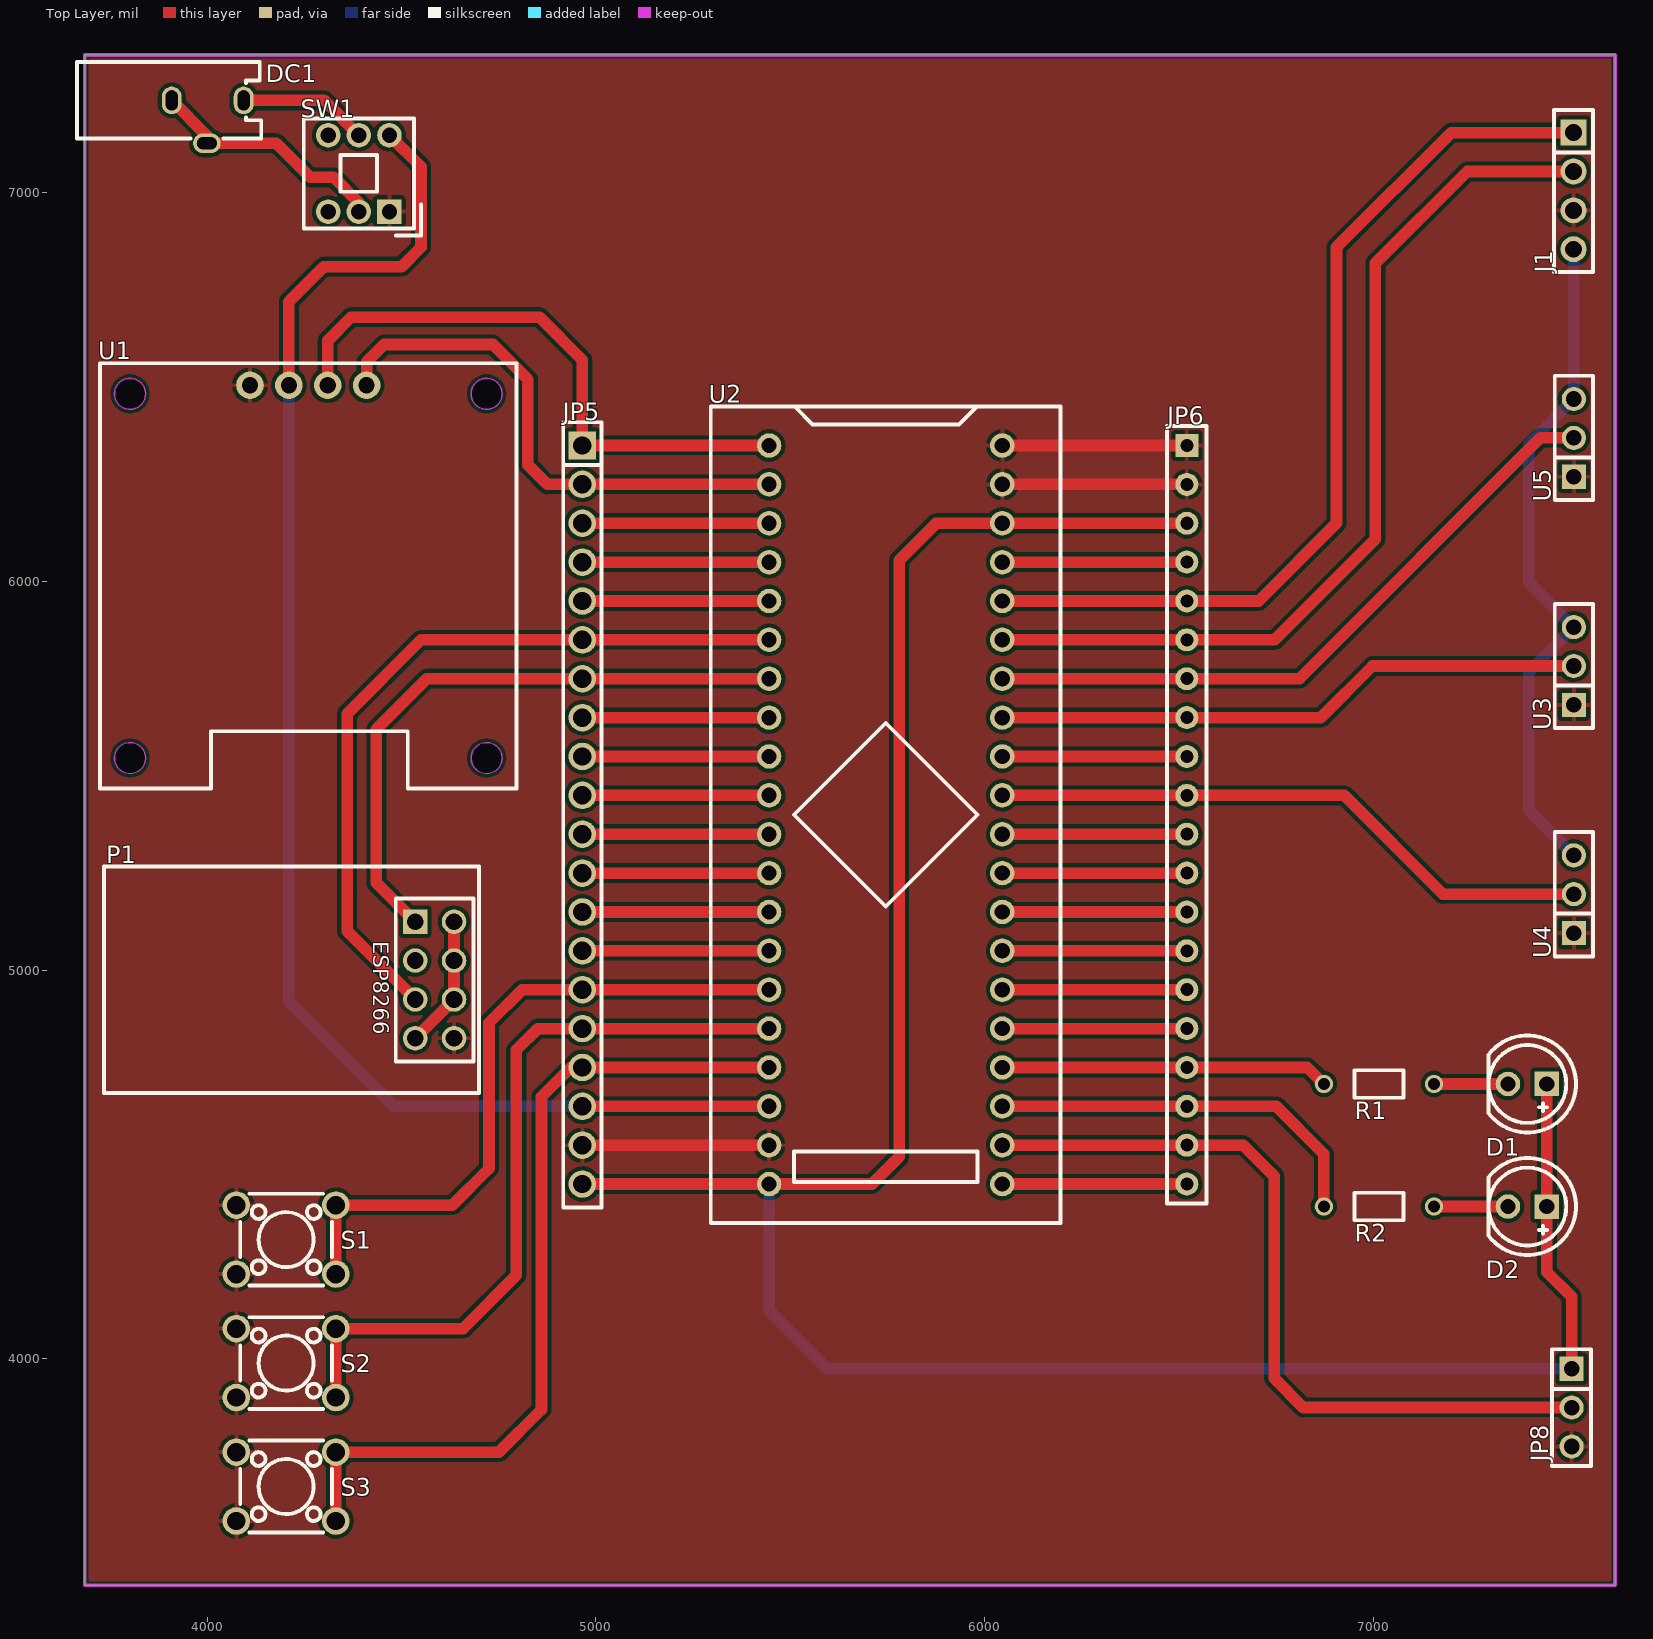
[diagram p0: Top Layer view]
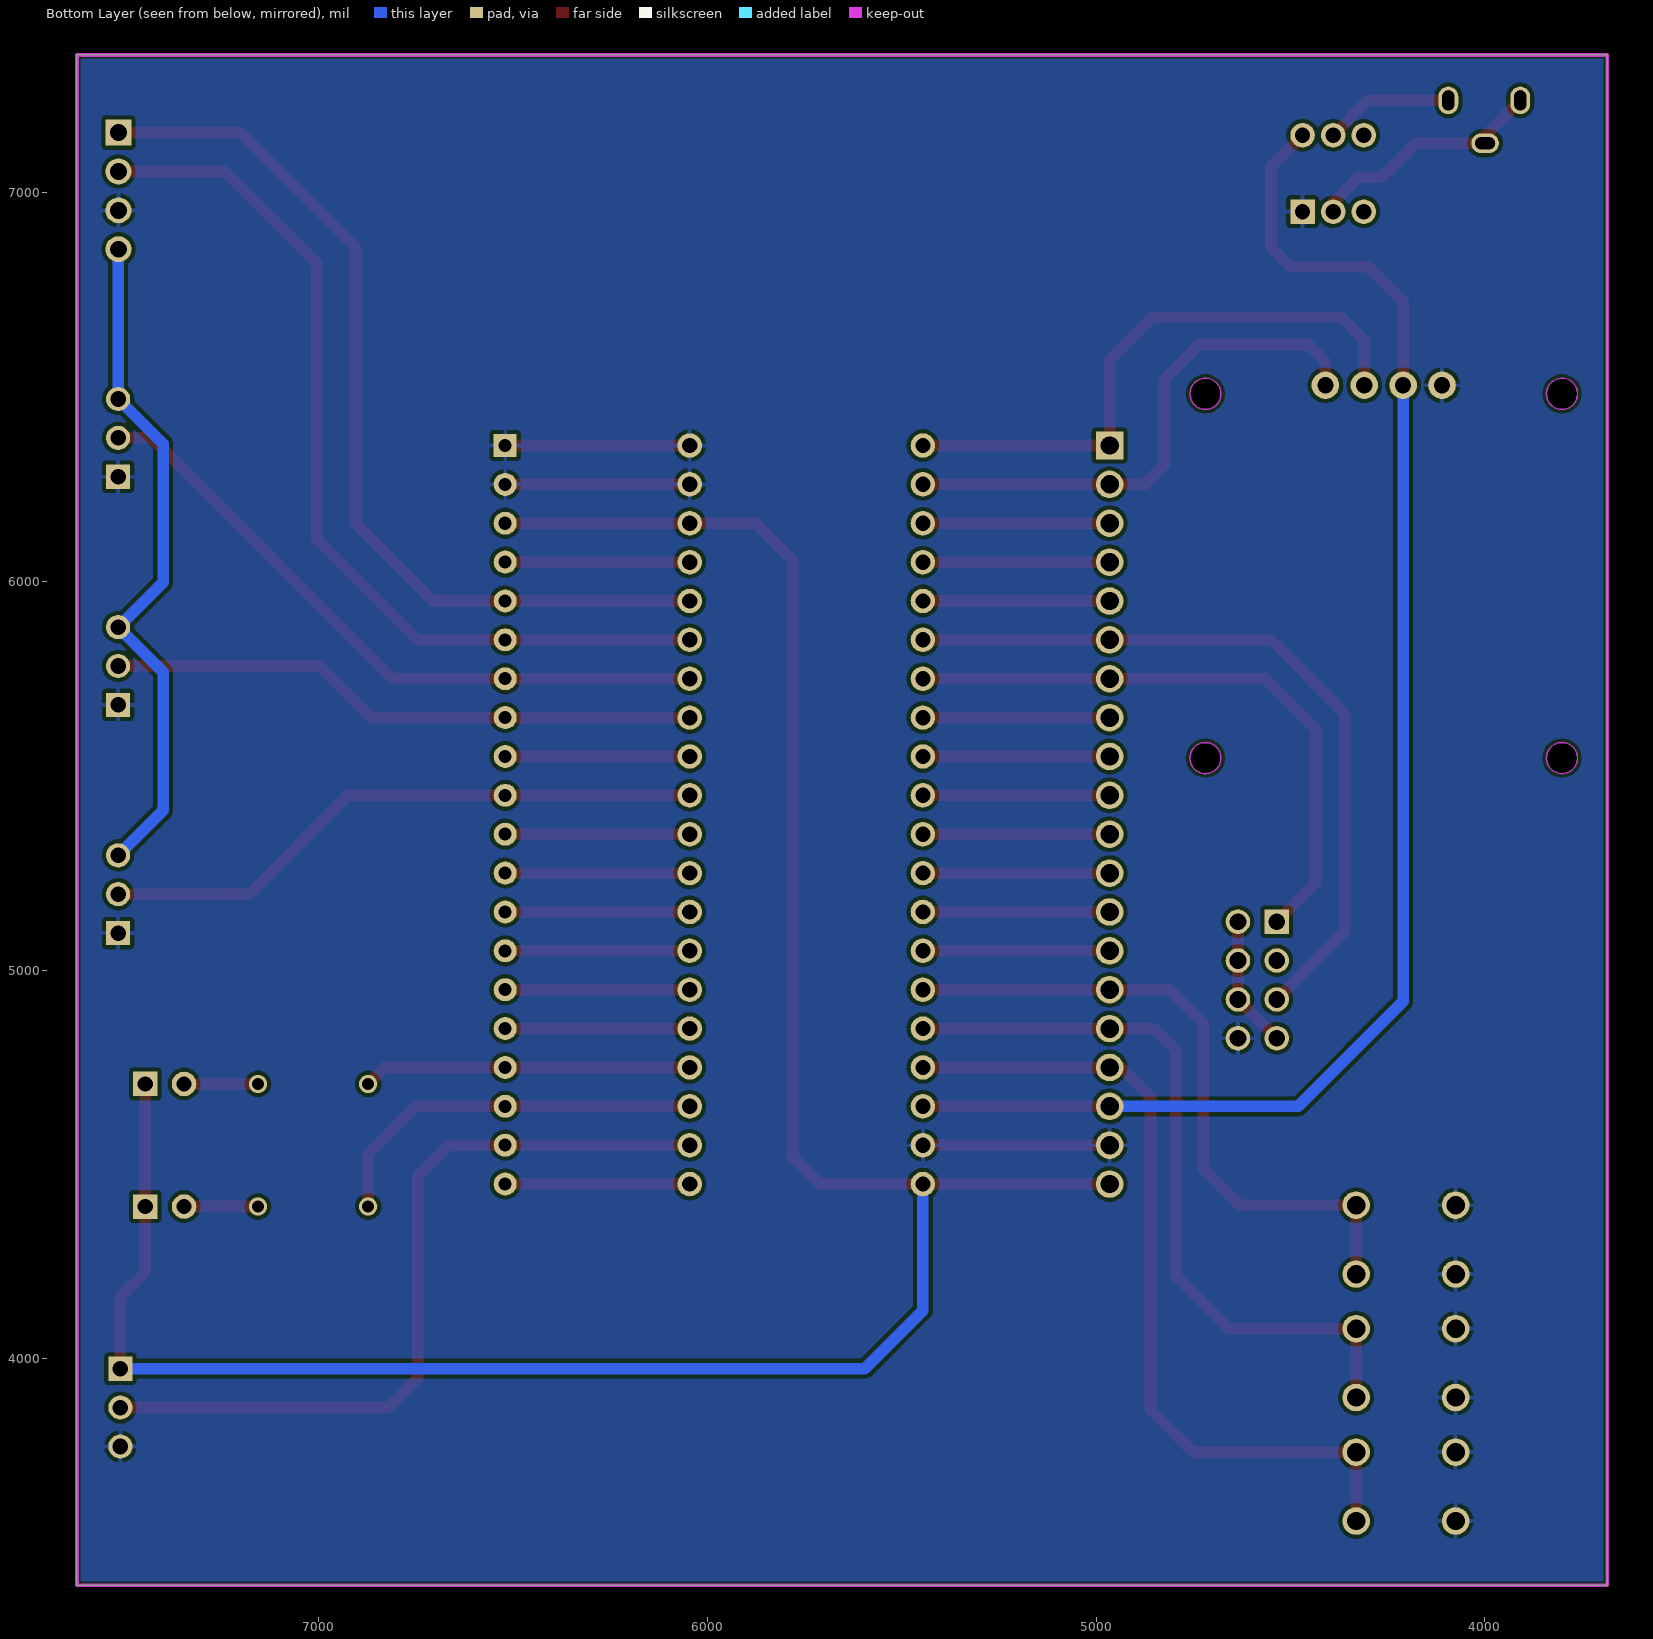
[diagram p1: Bottom Layer view, seen from below]
# Altium PCB MISC61251.pcbdoc
Units mil, origin at the board's own origin, x right, y up, seen from the top; angles counter-clockwise.
Board outline 3937.01 x 3937.01 mil, 2 copper layers (Top Layer, Bottom Layer), stack 62.206 mil thick; 19 components, 43 nets, 137 pads, 0 vias.

## Layer stack, top to bottom
Top Solder Mask Layer: solder mask 0.394, Dk 3.3
Top Layer: signal copper 1.379
Dielectric1: surface 59.449, FR4, Dk 4.5
Bottom Layer: signal copper 1.378
Bottom Solder Mask Layer: solder mask 0.394, Dk 3.3

## Board outline
3685,7355 3685,3417.99 7622.01,3417.99 7622.01,7355

## Design rules (kind name [scope] priority, off if disabled: settings)
BoardOutlineClearance copperThickness2oz_1 [All] p2 off: genericclearance=7.99 ignorepadtopadclearanceinfootprint=FALSE except(0: Arc-SplitContinuation Track-SplitContinuation SMDPad-SplitContinuation THPad-SplitContinuation Via-SplitContinuation Fill-SplitContinuation Region-SplitContinuation Poly-SplitContinuation Text-SplitContinuation Hole-SplitContinuation; 5.98: Arc-CutoutEdge SMDPad-CutoutEdge THPad-CutoutEdge Via-CutoutEdge Fill-CutoutEdge Region-CutoutEdge Text-CutoutEdge; 6.93: Hole-OutlineEdge Hole-CutoutEdge; 10: Poly-OutlineEdge Poly-CutoutEdge; 11.81: Arc-OutlineEdge Track-OutlineEdge SMDPad-OutlineEdge THPad-OutlineEdge Via-OutlineEdge Fill-OutlineEdge Region-OutlineEdge Text-OutlineEdge Track-CutoutEdge)
BoardOutlineClearance copperThickness1oz_1 [All] p4: genericclearance=4.02 ignorepadtopadclearanceinfootprint=FALSE except(0: Arc-SplitContinuation Track-SplitContinuation SMDPad-SplitContinuation THPad-SplitContinuation Via-SplitContinuation Fill-SplitContinuation Region-SplitContinuation Poly-SplitContinuation Text-SplitContinuation Hole-SplitContinuation; 6: SMDPad-CutoutEdge THPad-CutoutEdge Via-CutoutEdge Fill-CutoutEdge Region-CutoutEdge Text-CutoutEdge; 6.93: Hole-OutlineEdge Hole-CutoutEdge; 10: Poly-OutlineEdge Poly-CutoutEdge; 11.8: Arc-OutlineEdge Track-OutlineEdge SMDPad-OutlineEdge THPad-OutlineEdge Via-OutlineEdge Fill-OutlineEdge Region-OutlineEdge Text-OutlineEdge; 11.81: Arc-CutoutEdge Track-CutoutEdge)
Clearance copperThickness2oz [All] p1 off: gap=7.99 ignorepadtopadclearanceinfootprint=FALSE except(5.98: SMDPad-Track SMDPad-SMDPad THPad-Track SMDPad-THPad THPad-THPad Track-Via SMDPad-Via THPad-Via Via-Via Fill-Track Region-Track Fill-SMDPad Region-SMDPad Fill-THPad Region-THPad Fill-Via Region-Via Fill-Fill Fill-Region Region-Region Arc-Track Arc-SMDPad Arc-THPad Arc-Via Fill-Arc Region-Arc Arc-Arc Text-Track SMDPad-Text Text-THPad Text-Via Fill-Text Region-Text Arc-Text Text-Text; 6.93: Hole-Track Hole-SMDPad Hole-THPad Hole-Via Fill-Hole Region-Hole Hole-Arc Hole-Text; 10: Poly-Track Poly-SMDPad Poly-THPad Poly-Via Poly-Fill Poly-Region Poly-Poly Poly-Arc Poly-Text Poly-Hole)
Clearance copperThickness1oz [All] p3: gap=4.02 ignorepadtopadclearanceinfootprint=FALSE except(5.98: SMDPad-Track SMDPad-SMDPad THPad-Track SMDPad-THPad THPad-THPad Track-Via SMDPad-Via THPad-Via Via-Via Fill-Track Region-Track Fill-SMDPad Region-SMDPad Fill-THPad Region-THPad Fill-Via Region-Via Fill-Fill Fill-Region Region-Region; 6: Arc-Track Arc-SMDPad Arc-THPad Arc-Via Fill-Arc Region-Arc Arc-Arc Text-Track SMDPad-Text Text-THPad Text-Via Fill-Text Region-Text Arc-Text Text-Text; 6.93: Hole-Track Hole-SMDPad Hole-THPad Hole-Via Fill-Hole Region-Hole Hole-Arc Hole-Text; 10: Poly-Track Poly-SMDPad Poly-THPad Poly-Via Poly-Fill Poly-Region Poly-Poly Poly-Arc Poly-Text Poly-Hole)
DiffPairsRouting differentialPair [All] p1: maxlimit=6 minlimit=6 mostfreqgap=6 toplayer_minwidth=5 toplayer_prefwidth=10 toplayer_maxwidth=100 toplayer_mingap=6 toplayer_prefgap=6 toplayer_maxgap=6 bottomlayer_minwidth=5 bottomlayer_prefwidth=10 bottomlayer_maxwidth=100 bottomlayer_mingap=6 bottomlayer_prefgap=6 bottomlayer_maxgap=6 maxuncoupledlength=10
HoleToHoleClearance otherClearance [All] p1: gap=11.81 allowstackedmicrovias=TRUE
Length netLength [All] p1: minlimit=0 maxlimit=0
MatchedLengths netLengthTolerance [All] p1: tolerance=1000
PasteMaskExpansion pasteMaskExpansion [All] p1: expansion=0
PlaneConnect innerPlane [All] p1: planeconnectstyle=Relief reliefexpansion=20 reliefentries=4 reliefconductorwidth=10 reliefairgap=10
PolygonConnect copperRegion [(InNet('GND'))] p1: connectstyle=Relief reliefconductorwidth=10 reliefentries=4 polygonreliefangle="90 Angle" airgapwidth=10 via.connectstyle=Relief via.reliefconductorwidth=10 via.reliefentries=4 via.polygonreliefangle="90 Angle" via.airgapwidth=10
RoutingVias viaSize [All] p1: holewidth=12.01 width=24.02 viastyle="Through Hole" minholewidth=11.81 minwidth=19.68 maxholewidth=248.03 maxwidth=393.7
SolderMaskExpansion solderMaskExpansion [IsVia] p1: expansion=-1000 istentingtop=TRUE
SolderMaskExpansion solderMaskExpansion [All] p2: expansion=2 istentingtop=FALSE
Width copperThickness2oz_2 [All] p1 off: maxlimit=100 minlimit=8 preferedwidth=10
Width copperThickness1oz_2 [All] p2: maxlimit=100 minlimit=5 preferedwidth=10

## Components (designator, comment, footprint, x,y, rotation, side; value= is the part's Value field where it differs from the comment)
D1 "led" LED-TH_5mm 7396.22,4707.52 r180 top
D2 "led" LED-TH_5mm 7396.22,4392.2 r180 top
DC1 "DC002-1.3" DC-IN-TH_DC002-1.3 4001.22,7182.72 r270 top
J1 "" HDR-TH_4P-P2.54-V-F 7515,7005 r270 top
JP5 "HDR-1X20" HDR-TH_20P-P2.54-V-F 4965,5400 r270 top
JP6 "HDR-1X20" HDR-TH_20P-P2.54-V-F-6 6520,5400 r270 top
JP8 "HDR-1X3" HDR-TH_3P-P2.54-V-F-4 7510,3875 r270 top
P1 "" ESP8266-1 4585,4975 r270 top
R1 "Res2" Res_1/8W 7014.4,4709.99 r180 top
R2 "Res2" Res_1/8W 7014.4,4394.68 r180 top
S1 "key_4" SW-TH_4P-L6.0-W6.0-P4.50-LS6.5 4203.02,4307.03 r180 top
S2 "key_4" SW-TH_4P-L6.0-W6.0-P4.50-LS6.5 4203.02,3989.4 r180 top
S3 "key_4" SW-TH_4P-L6.0-W6.0-P4.50-LS6.5 4203.02,3671.76 r180 top
SW1 "Self-lock button" SW-TH_6P-L7.0-W7.0-P2.00 4390,7050 r270 top
U1 "OLED" OLED-TH_L27.8-W27.2-P2.54_C9900033791 4260,6505 r0 top
U2 "ST32F103C8T6" CONN-TH_L53.3-W22.9_STM32F103C8T6-CARD 5745.45,5400 r270 top
U3 "" HDR-TH_3P-P2.54-V-F 7515.79,5782.68 r90 top
U4 "" HDR-TH_3P-P2.54-V-F 7515.79,5195.73 r90 top
U5 "DHT11" HDR-TH_3P-P2.54-V-F 7515.79,6369.63 r90 top

## Footprints (in the part's own frame and the unit in brackets; to place one, negate y for a bottom-side part, rotate by r counter-clockwise, add the part's x,y. Pads: shape width x height; smd on the part's side, far side on the other; paste and mask are expansions set on the pad)
CONN-TH_L53.3-W22.9_STM32F103C8T6-CARD [mm]
  round 1.6 hole 1: 1(-24.13,-7.62) 2(-21.59,-7.62) 3(-19.05,-7.62) 4(-16.51,-7.62) 5(-13.97,-7.62) 6(-11.43,-7.62) 7(-8.89,-7.62) 8(-6.35,-7.62) 9(-3.81,-7.62) 10(-1.27,-7.62) 11(1.27,-7.62) 12(3.81,-7.62) 13(6.35,-7.62) 14(8.89,-7.62) 15(11.43,-7.62) 16(13.97,-7.62) 17(16.51,-7.62) 18(19.05,-7.62) 19(21.59,-7.62) 20(24.13,-7.62) 21(24.13,7.62) 22(21.59,7.62) 23(19.05,7.62) 24(16.51,7.62) 25(13.97,7.62) 26(11.43,7.62) 27(8.89,7.62) 28(6.35,7.62) 29(3.81,7.62) 30(1.27,7.62) 31(-1.27,7.62) 32(-3.81,7.62) 33(-6.35,7.62) 34(-8.89,7.62) 35(-11.43,7.62) 36(-13.97,7.62) 37(-16.51,7.62) 38(-19.05,7.62) 39(-21.59,7.62) 40(-24.13,7.62)
  silkscreen extent -26.67,-11.43 26.67,11.43
DC-IN-TH_DC002-1.3 [mm]
  oval 1.8x1.3 hole 0.8 slot 1.3 at 0 deg paste+0 mask+0.05: 1(-1.4,2.35) 3(-1.4,-2.35)
  oval 1.3x1.8 hole 0.8 slot 1.3 at 90 deg paste+0 mask+0.05: 2(1.4,-0.05)
  silkscreen extent -3.9,-8.55 1.1,3.5
ESP8266-1 [mm]
  rect 1.6x1.6 hole 1.1: 1(-3.81,-1.27)
  round 1.6 hole 1.1: 2(-3.81,1.27) 3(-1.27,-1.27) 4(-1.27,1.27) 5(1.27,-1.27) 6(1.27,1.27) 7(3.81,-1.27) 8(3.81,1.27)
  silkscreen extent -7.42,-21.6 7.38,2.9
HDR-TH_3P-P2.54-V-F [mil]
  rect 62x62 hole 40.16: 1(-100,0)
  round 62 hole 40.16: 2(0,0) 3(100,0)
  silkscreen extent -160,-49 160,49
HDR-TH_3P-P2.54-V-F-4 [mil]
  rect 62x62 hole 40.16: 1(-100,0)
  round 62 hole 40.16: 2(0,0) 3(100,0)
  silkscreen extent -150,-50 150,50
HDR-TH_4P-P2.54-V-F [mm]
  rect 1.7x1.7 hole 1.1: 1(-3.81,0)
  round 1.7 hole 1.1: 2(-1.27,0) 3(1.27,0) 4(3.81,0)
  silkscreen extent -5.29,-1.27 5.29,1.27
HDR-TH_20P-P2.54-V-F [mm]
  rect 1.8x1.8 hole 1.2: 1(-24.13,0)
  round 1.8 hole 1.2: 2(-21.59,0) 3(-19.05,0) 4(-16.51,0) 5(-13.97,0) 6(-11.43,0) 7(-8.89,0) 8(-6.35,0) 9(-3.81,0) 10(-1.27,0) 11(1.27,0) 12(3.81,0) 13(6.35,0) 14(8.89,0) 15(11.43,0) 16(13.97,0) 17(16.51,0) 18(19.05,0) 19(21.59,0) 20(24.13,0)
  silkscreen extent -25.65,-1.25 25.65,1.25
HDR-TH_20P-P2.54-V-F-6 [mm]
  rect 1.5x1.5 hole 0.85 paste+0 mask+0.05: 1(-24.13,0)
  round 1.5 hole 0.85 paste+0 mask+0.05: 2(-21.59,0) 3(-19.05,0) 4(-16.51,0) 5(-13.97,0) 6(-11.43,0) 7(-8.89,0) 8(-6.35,0) 9(-3.81,0) 10(-1.27,0) 11(1.27,0) 12(3.81,0) 13(6.35,0) 14(8.89,0) 15(11.43,0) 16(13.97,0) 17(16.51,0) 18(19.05,0) 19(21.59,0) 20(24.13,0)
  silkscreen extent -25.4,-1.3 25.4,1.3
LED-TH_5mm [mm]
  rect 1.6x1.6 hole 1 paste+0 mask+0.051: 1(-1.27,0)
  round 1.6 hole 1 paste+0 mask+0.051: 2(1.27,0)
  silkscreen extent -3.17,-3.17 2.54,3.17
OLED-TH_L27.8-W27.2-P2.54_C9900033791 [mm]
  round 1.8 hole 1.05 paste+0 mask+0.05: 1(-3.81,0) 2(-1.27,0) 3(1.27,0) 4(3.81,0)
  Board Outline Layer circle w0.003: c-11.65,-0.56 r1.016
  Board Outline Layer circle w0.003: c11.65,-0.56 r1.016
  Board Outline Layer circle w0.003: c-11.65,-24.36 r1.016
  Board Outline Layer circle w0.003: c11.65,-24.36 r1.016
  Board Outline Layer region: -10.634,-0.56 -10.735,-1.001 -11.016,-1.354 -11.424,-1.551 -11.876,-1.551 -12.283,-1.354 -12.565,-1.001 -12.666,-0.56 -12.666,-0.56 -12.565,-0.119 -12.283,0.234 -11.876,0.431 -11.424,0.431 -11.016,0.234 -10.735,-0.119 -10.634,-0.56
  Board Outline Layer region: -10.634,-0.56 -10.643,-0.698 -10.672,-0.834 -10.718,-0.965 -10.782,-1.088 -10.862,-1.201 -10.956,-1.303 -11.064,-1.39 -11.183,-1.462 -11.31,-1.517 -11.443,-1.555 -11.581,-1.574 -11.719,-1.574 -11.857,-1.555 -11.99,-1.517 -12.117,-1.462 -12.236,-1.39 -12.343,-1.303 -12.438,-1.201 -12.518,-1.088 -12.582,-0.965 -12.628,-0.834 -12.656,-0.698 -12.666,-0.56 -12.656,-0.422 -12.628,-0.286 -12.582,-0.155 -12.518,-0.032 -12.438,0.081 -12.343,0.183 -12.236,0.27 -12.117,0.342 -11.99,0.397 -11.857,0.435 -11.719,0.454 -11.581,0.454 -11.443,0.435 -11.31,0.397 -11.183,0.342 -11.064,0.27 -10.956,0.183 -10.862,0.081 -10.782,-0.032 -10.718,-0.155 -10.672,-0.286 -10.643,-0.422
  Board Outline Layer region: 12.666,-0.56 12.565,-1.001 12.283,-1.354 11.876,-1.551 11.424,-1.551 11.017,-1.354 10.735,-1.001 10.634,-0.56 10.634,-0.56 10.735,-0.119 11.017,0.234 11.424,0.431 11.876,0.431 12.283,0.234 12.565,-0.119 12.666,-0.56
  Board Outline Layer region: 12.666,-0.56 12.657,-0.698 12.628,-0.834 12.582,-0.965 12.518,-1.088 12.438,-1.201 12.343,-1.303 12.236,-1.39 12.117,-1.462 11.99,-1.517 11.857,-1.555 11.719,-1.574 11.581,-1.574 11.443,-1.555 11.31,-1.517 11.183,-1.462 11.064,-1.39 10.957,-1.303 10.862,-1.201 10.782,-1.088 10.718,-0.965 10.672,-0.834 10.643,-0.698 10.634,-0.56 10.643,-0.422 10.672,-0.286 10.718,-0.155 10.782,-0.032 10.862,0.081 10.957,0.183 11.064,0.27 11.183,0.342 11.31,0.397 11.443,0.435 11.581,0.454 11.719,0.454 11.857,0.435 11.99,0.397 12.117,0.342 12.236,0.27 12.343,0.183 12.438,0.081 12.518,-0.032 12.582,-0.155 12.628,-0.286 12.657,-0.422
  Board Outline Layer region: -10.634,-24.36 -10.735,-24.801 -11.016,-25.154 -11.424,-25.35 -11.876,-25.35 -12.283,-25.154 -12.565,-24.801 -12.666,-24.36 -12.666,-24.36 -12.565,-23.919 -12.283,-23.566 -11.876,-23.369 -11.424,-23.369 -11.016,-23.566 -10.735,-23.919 -10.634,-24.36
  Board Outline Layer region: -10.634,-24.36 -10.643,-24.498 -10.672,-24.634 -10.718,-24.765 -10.782,-24.888 -10.862,-25.001 -10.956,-25.102 -11.064,-25.19 -11.183,-25.262 -11.31,-25.317 -11.443,-25.355 -11.581,-25.374 -11.719,-25.374 -11.857,-25.355 -11.99,-25.317 -12.117,-25.262 -12.236,-25.19 -12.343,-25.102 -12.438,-25.001 -12.518,-24.888 -12.582,-24.765 -12.628,-24.634 -12.656,-24.498 -12.666,-24.36 -12.656,-24.222 -12.628,-24.086 -12.582,-23.955 -12.518,-23.832 -12.438,-23.719 -12.343,-23.617 -12.236,-23.53 -12.117,-23.458 -11.99,-23.403 -11.857,-23.365 -11.719,-23.346 -11.581,-23.346 -11.443,-23.365 -11.31,-23.403 -11.183,-23.458 -11.064,-23.53 -10.956,-23.617 -10.862,-23.719 -10.782,-23.832 -10.718,-23.955 -10.672,-24.086 -10.643,-24.222
  Board Outline Layer region: 12.666,-24.36 12.565,-24.801 12.283,-25.154 11.876,-25.35 11.424,-25.35 11.017,-25.154 10.735,-24.801 10.634,-24.36 10.634,-24.36 10.735,-23.919 11.017,-23.566 11.424,-23.369 11.876,-23.369 12.283,-23.566 12.565,-23.919 12.666,-24.36
  Board Outline Layer region: 12.666,-24.36 12.657,-24.498 12.628,-24.634 12.582,-24.765 12.518,-24.888 12.438,-25.001 12.343,-25.102 12.236,-25.19 12.117,-25.262 11.99,-25.317 11.857,-25.355 11.719,-25.374 11.581,-25.374 11.443,-25.355 11.31,-25.317 11.183,-25.262 11.064,-25.19 10.957,-25.102 10.862,-25.001 10.782,-24.888 10.718,-24.765 10.672,-24.634 10.643,-24.498 10.634,-24.36 10.643,-24.222 10.672,-24.086 10.718,-23.955 10.782,-23.832 10.862,-23.719 10.957,-23.617 11.064,-23.53 11.183,-23.458 11.31,-23.403 11.443,-23.365 11.581,-23.346 11.719,-23.346 11.857,-23.365 11.99,-23.403 12.117,-23.458 12.236,-23.53 12.343,-23.617 12.438,-23.719 12.518,-23.832 12.582,-23.955 12.628,-24.086 12.657,-24.222
  Multi-Layer board cut-out: -10.634,-0.56 -10.735,-1.001 -11.016,-1.354 -11.424,-1.551 -11.876,-1.551 -12.283,-1.354 -12.565,-1.001 -12.666,-0.56 -12.666,-0.56 -12.565,-0.119 -12.283,0.234 -11.876,0.431 -11.424,0.431 -11.016,0.234 -10.735,-0.119 -10.634,-0.56
  Multi-Layer board cut-out: 12.666,-0.56 12.565,-1.001 12.283,-1.354 11.876,-1.551 11.424,-1.551 11.017,-1.354 10.735,-1.001 10.634,-0.56 10.634,-0.56 10.735,-0.119 11.017,0.234 11.424,0.431 11.876,0.431 12.283,0.234 12.565,-0.119 12.666,-0.56
  Multi-Layer board cut-out: -10.634,-24.36 -10.735,-24.801 -11.016,-25.154 -11.424,-25.35 -11.876,-25.35 -12.283,-25.154 -12.565,-24.801 -12.666,-24.36 -12.666,-24.36 -12.565,-23.919 -12.283,-23.566 -11.876,-23.369 -11.424,-23.369 -11.016,-23.566 -10.735,-23.919 -10.634,-24.36
  Multi-Layer board cut-out: 12.666,-24.36 12.565,-24.801 12.283,-25.154 11.876,-25.35 11.424,-25.35 11.017,-25.154 10.735,-24.801 10.634,-24.36 10.634,-24.36 10.735,-23.919 11.017,-23.566 11.424,-23.369 11.876,-23.369 12.283,-23.566 12.565,-23.919 12.666,-24.36
  silkscreen extent -13.6,-26.36 13.6,1.44
Res_1/8W [mil]
  round 47.2 hole 31.5 paste+0 mask+2: 1(-141.7,2.48) 2(141.7,2.48)
  silkscreen extent -63,-33 63,38
SW-TH_4P-L6.0-W6.0-P4.50-LS6.5 [mm]
  round 1.8 hole 1.2: 1(-3.25,2.25) 2(3.25,2.25) 3(-3.25,-2.25) 4(3.25,-2.25)
  silkscreen extent -3,-3 3,3
SW-TH_6P-L7.0-W7.0-P2.00 [mm]
  rect 1.6x1.6 hole 1: 1(2.5,2)
  round 1.6 hole 1: 2(2.5,0) 3(2.5,-2) 4(-2.5,2) 5(-2.5,0) 6(-2.5,-2)
  silkscreen extent -3.6,-3.6 4.06,4.06

## Nets (pads, with @x,y where several pads share a name; then routed paths per layer and width w, separated by ;. In a path a pad name is that pad's centre, name@x,y a point inside that pad or via, vN(x,y) a via of type N, cw(c..) or ccw(c..) an arc to the next point about the centre after c; other vN are vias at no path point)
3.3V: P1.2 P1.4 P1.6 P1.7 | length 341.4
  Top Layer w30: P1.7 P1.6 P1.4 P1.2
$2N41: D1.2 R1.1 | length 190.1
  Top Layer w30: R1.1 D1.2
$2N43: D2.2 R2.1 | length 190.1
  Top Layer w30: R2.1 D2.2
$2N54: JP6.4 U2.37 | length 479.5
  Top Layer w30: U2.37 JP6.4@6525,6050
$2N55: JP6.20 U2.21 | length 479.5
  Top Layer w30: U2.21 JP6.20@6525,4450
+3: D1.1 D2.1 JP5.20 JP6.3 JP8.1 U2.20 U2.38 | length 6374.2
  Top Layer w30: JP5.20 U2.20 5710,4450 5780,4520 5780,6055 5875,6150 U2.38 JP6.3@6525,6150 ; D1.1 D2.1 7446.22,4223.78 7510,4160 JP8.1
  Bottom Layer w30: U2.20 5445.45,4124.55 5595,3975 JP8.1
+5: JP5.18 SW1.4 U1.2 U2.18 | length 3867.4
  Top Layer w30: U1.2 4210,6720 4300,6810 4500,6810 4550,6860 4550,7067.16 SW1.4 ; JP5.18 U2.18
  Bottom Layer w30: U1.2 4210,4920 4480,4650 JP5.18
DC_GND: DC1.2 DC1.3 SW1.2 | length 625.1
  Top Layer w30: DC1.3 3999.25,7147.29 DC1.2 4177.39,7127.61 4265,7040 4325,7040 4390,6975 SW1.2
DC_VCC: DC1.1 SW1.5 | length 333.3
  Top Layer w30: DC1.1 4300.59,7237.84 SW1.5
GND: J1.3 JP5.19 JP6.1 JP6.2 JP8.3 P1.8 S1.2 S1.4 S2.2 S2.4 S3.2 S3.4 SW1.1 U1.1 U2.19 U2.39 U2.40 U3.1 U4.1 U5.1 | length 1439.5
  Top Layer w30: JP5.19 U2.19 ; U2.39 JP6.2@6525,6250 ; U2.40 JP6.1@6525,6350
PA0: JP6.16 U2.25 | length 479.5
  Top Layer w30: U2.25 JP6.16@6525,4850
PA1: JP6.15 U2.26 | length 479.5
  Top Layer w30: U2.26 JP6.15@6525,4950
PA2: JP6.14 U2.27 | length 479.5
  Top Layer w30: U2.27 JP6.14@6525,5050
PA3: JP6.13 U2.28 | length 479.5
  Top Layer w30: U2.28 JP6.13@6525,5150
PA4: JP6.12 U2.29 | length 479.5
  Top Layer w30: U2.29 JP6.12@6525,5250
PA5: JP6.11 U2.30 | length 479.5
  Top Layer w30: U2.30 JP6.11@6525,5350
PA6: JP6.10 U2.31 U4.2 | length 1575.7
  Top Layer w30: U2.31 JP6.10 6925,5450 7179.27,5195.73 U4.2
PA7: JP6.9 U2.32 | length 479.5
  Top Layer w30: U2.32 JP6.9@6525,5550
PA8: JP5.5 U2.5 | length 480.5
  Top Layer w30: JP5.5 U2.5
PA9: JP5.6 P1.5 U2.6 | length 1971.6
  Top Layer w30: P1.5 4360,5100 4360,5660 4550,5850 JP5.6 U2.6
PA10: JP5.7 P1.1 U2.7 | length 1600.7
  Top Layer w30: P1.1 4435,5225 4435,5620 4565,5750 JP5.7 U2.7
PA11: JP5.8 U2.8 | length 480.5
  Top Layer w30: JP5.8 U2.8
PA12: JP5.9 U2.9 | length 480.5
  Top Layer w30: JP5.9 U2.9
PA15: JP5.10 U2.10 | length 480.5
  Top Layer w30: JP5.10 U2.10
PB0: JP6.8 U2.33 U3.2 | length 1525.3
  Top Layer w30: U2.33 JP6.8 6865,5650 6997.68,5782.68 U3.2
PB1: JP6.7 U2.34 U5.2 | length 1727
  Top Layer w30: U2.34 JP6.7 6810,5750 7429.63,6369.63 U5.2
PB3: JP5.11 U2.11 | length 480.5
  Top Layer w30: JP5.11 U2.11
PB4: JP5.12 U2.12 | length 480.5
  Top Layer w30: JP5.12 U2.12
PB5: JP5.13 U2.13 | length 480.5
  Top Layer w30: JP5.13 U2.13
PB6: JP5.14 U2.14 | length 480.5
  Top Layer w30: JP5.14 U2.14
PB7: JP5.15 S1.1 S1.3 U2.15 | length 1740.9
  Top Layer w30: S1.1 S1.3 4630.61,4395.61 4725,4490 4725,4865 4810,4950 JP5.15 U2.15
PB8: JP5.16 S2.1 S2.3 U2.16 | length 1951.2
  Top Layer w30: S2.1 S2.3 4657.98,4077.98 4795,4215 4795,4795 4850,4850 JP5.16 U2.16
PB9: JP5.17 S3.1 S3.3 U2.17 | length 2173.1
  Top Layer w30: S3.1 S3.3 4750.34,3760.34 4860,3870 4860,4675 4935,4750 JP5.17 U2.17
PB10: J1.2 JP6.6 U2.35 | length 2384.6
  Top Layer w30: U2.35 6746.42,5850 7005,6108.58 7005,6818.58 7241.42,7055 J1.2
PB11: J1.1 JP6.5 U2.36 | length 2384.6
  Top Layer w30: U2.36 6705,5950 6905,6150 6905,6860 7200,7155 J1.1
PB12: JP5.1 U1.3 U2.1 | length 1540.9
  Top Layer w30: U1.3 4310,6620 4370,6680 4855,6680 4965,6570 JP5.1 U2.1
PB13: JP5.2 U1.4 U2.2 | length 1392.1
  Top Layer w30: U1.4 4410,6565 4455,6610 4735,6610 4825,6520 4825,6300 4875,6250 JP5.2 U2.2
PB14: JP5.3 U2.3 | length 480.5
  Top Layer w30: JP5.3 U2.3
PB15: JP5.4 U2.4 | length 480.5
  Top Layer w30: JP5.4 U2.4
PC13: JP6.19 JP8.2 U2.22 | length 2048.7
  Top Layer w30: U2.22 JP6.19 6665,4550 6745,4470 6745,3950 6820,3875 JP8.2
PC14: JP6.18 R2.2 U2.23 | length 1013.2
  Top Layer w30: U2.23 JP6.18 6750,4650 6872.7,4527.3 R2.2
PC15: JP6.17 R1.2 U2.24 | length 844.8
  Top Layer w30: U2.24 JP6.17 6830.22,4750 R1.2
VCC: J1.4 U3.3 U4.3 U5.3 | length 1751.4
  Bottom Layer w30: J1.4 7515.79,6854.21 U5.3 7400,6353.84 7400,5998.47 U3.3 7400,5766.89 7400,5411.52 U4.3
pads on no net: P1.3 SW1.3 SW1.6

## Polygon pours and split planes (outlines as drawn)
GND on Top Layer (solid, remove dead copper, pour order 0): 3000,7770 3000,3000 8180,3000 8180,7770
GND on Bottom Layer (solid, remove dead copper, pour order 2): 3475,7760 3475,3050 7985,3050 7985,7760

## Keep-outs
Board Outline Layer:
  the board outline again, w10